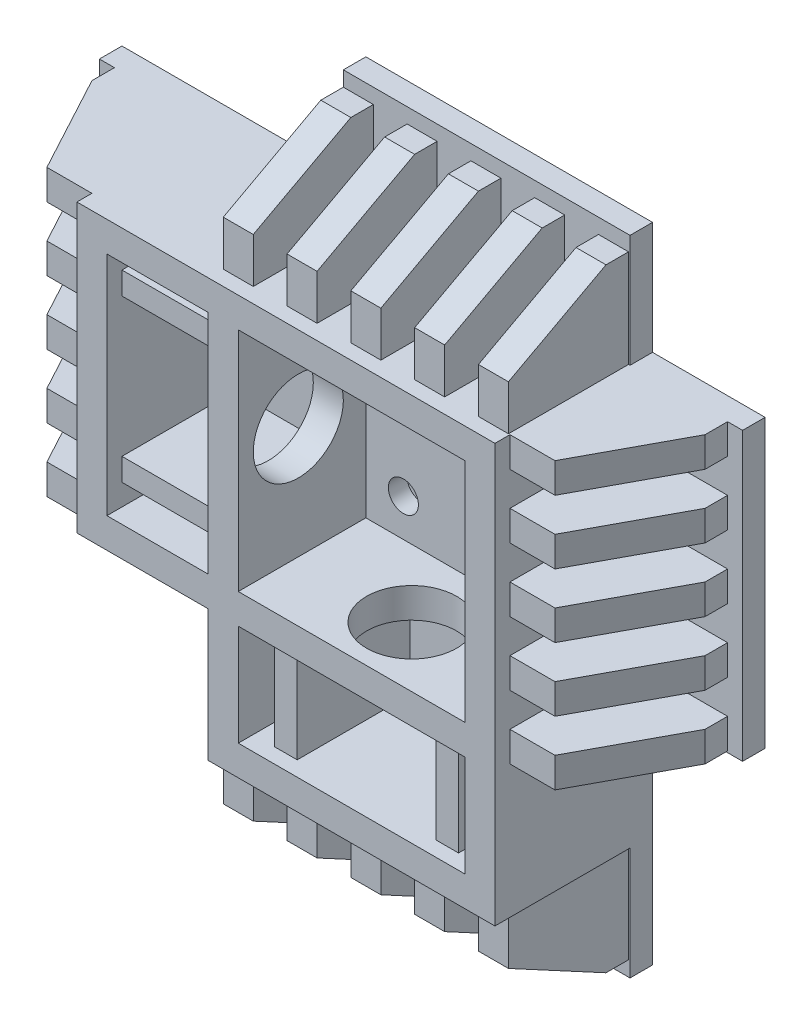
SolidWorks part; units mm, degrees
ref_plane "Front Plane" through (0, 0, 0) normal (0, 0, 1) x (1, 0, 0)
ref_plane "Top Plane" through (0, 0, 0) normal (0, 1, 0) x (1, 0, 0)
ref_plane "Right Plane" through (0, 0, 0) normal (1, 0, 0) x (0, 0, -1)
sketch "Sketch1" plane through (0, 0, 0) normal (0, 0, 1) x (1, 0, 0)
  line L0 (278.5, -428.5) -> (278.5, -103.5)
  line L1 (278.5, 428.5) -> (-103.5, 428.5)
  line L2 (428.5, 278.5) -> (428.5, -103.5)
  line L3 (278.5, -428.5) -> (-103.5, -428.5)
  line L4 (-428.5, 278.5) -> (-428.5, -103.5)
  line L5 (428.5, 428.5) -> (-428.5, -428.5) construction
  line L6 (428.5, -428.5) -> (-428.5, 428.5) construction
  line L7 (278.5, -103.5) -> (428.5, -103.5)
  line L8 (-103.5, -103.5) -> (-103.5, -428.5)
  line L9 (-103.5, -103.5) -> (-428.5, -103.5)
  line L10 (-428.5, 278.5) -> (-103.5, 278.5)
  line L11 (-103.5, 278.5) -> (-103.5, 428.5)
  line L12 (278.5, 428.5) -> (278.5, 278.5)
  line L13 (278.5, 278.5) -> (428.5, 278.5)
  point P0 (0, 0)
  dimension "D1" = 857
  dimension "D2" = 857
  dimension "D3" = 325
  dimension "D4" = 150
  dimension "D5" = 325
  dimension "D6" = 150
extrude "Boss-Extrude1" add sketch "Sketch1" along normal blind 30
sketch "Sketch4" plane through (0, 0, 0) normal (0, 0, -1) x (-1, 0, 0)
  line L1 (-278.5, -278.5) -> (103.5, -278.5)
  line L2 (278.5, -103.5) -> (278.5, 278.5)
  line L3 (103.5, 278.5) -> (-278.5, 278.5)
  line L12 (-278.5, -428.5) -> (103.5, -428.5)
  line L13 (103.5, -428.5) -> (103.5, -103.5)
  line L14 (103.5, -103.5) -> (428.5, -103.5)
  line L15 (428.5, -103.5) -> (428.5, 278.5)
  line L16 (428.5, 278.5) -> (103.5, 278.5)
  line L17 (103.5, 278.5) -> (103.5, 428.5)
  line L18 (103.5, 428.5) -> (-278.5, 428.5)
  line L19 (-278.5, 428.5) -> (-278.5, 278.5)
  line L20 (-278.5, 278.5) -> (-428.5, 278.5)
  line L21 (-428.5, 278.5) -> (-428.5, -103.5)
  line L22 (-428.5, -103.5) -> (-278.5, -103.5)
  line L23 (-278.5, -103.5) -> (-278.5, -428.5)
  line L25 (103.5, -278.5) -> (103.5, -103.5)
  line L26 (103.5, -103.5) -> (278.5, -103.5)
  line L28 (278.5, 278.5) -> (103.5, 278.5)
  line L35 (-278.5, 278.5) -> (-278.5, -278.5)
  dimension "D1" = 0
extrude "Boss-Extrude2" add sketch "Sketch4" against normal blind 210
sketch "Sketch6" plane through (0, 0, 210) normal (0, 0, 1) x (1, 0, 0)
  line L0 (-278.5, 278.5) -> (278.5, 278.5) construction
  line L1 (238.5, 238.5) -> (-63.5, 238.5)
  line L2 (238.5, 238.5) -> (238.5, -63.5)
  line L3 (238.5, -63.5) -> (-63.5, -63.5)
  line L4 (-63.5, 238.5) -> (-63.5, -63.5)
  line L5 (238.5, 238.5) -> (-63.5, -63.5) construction
  line L6 (238.5, -63.5) -> (-63.5, 238.5) construction
  line L8 (278.5, 278.5) -> (278.5, -278.5) construction
  line L9 (-278.5, 278.5) -> (-278.5, -103.5) construction
  line L10 (-103.5, -63.5) -> (-238.5, -63.5)
  line L11 (-103.5, -63.5) -> (-103.5, 238.5)
  line L12 (-103.5, 238.5) -> (-238.5, 238.5)
  line L13 (-238.5, -63.5) -> (-238.5, 238.5)
  line L14 (-103.5, -63.5) -> (-238.5, 238.5) construction
  line L15 (-103.5, 238.5) -> (-238.5, -63.5) construction
  line L16 (278.5, -278.5) -> (-103.5, -278.5) construction
  line L17 (238.5, -103.5) -> (-63.5, -103.5)
  line L18 (238.5, -103.5) -> (238.5, -238.5)
  line L19 (238.5, -238.5) -> (-63.5, -238.5)
  line L20 (-63.5, -103.5) -> (-63.5, -238.5)
  line L21 (238.5, -103.5) -> (-63.5, -238.5) construction
  line L22 (238.5, -238.5) -> (-63.5, -103.5) construction
  line L23 (-103.5, -278.5) -> (-103.5, -103.5) construction
  point P0 (87.5, 87.5)
  point P7 (-171, 87.5)
  point P16 (87.5, -171)
  dimension "D1" = 302
  dimension "D2" = 302
  dimension "D3" = 40
  dimension "D4" = 40
  dimension "D5" = 40
  dimension "D6" = 40
  dimension "D7" = 40
  dimension "D8" = 40
  dimension "D9" = 40
  dimension "D10" = 40
extrude "Cut-Extrude3" cut sketch "Sketch6" against normal blind 170
sketch "Sketch7" plane through (-63.5, 0, 0) normal (1, 0, 0) x (0, 0, -1)
  line L0 (-210, 278.5) -> (-210, -278.5) construction
  circle A0 centre (-130, 87.5) radius 60
  dimension "D1" = 120
  dimension "D2" = 80
  dimension "D3" = 151
extrude "Cut-Extrude4" cut sketch "Sketch7" against normal blind 148
sketch "Sketch8" plane through (0, 0, 30) normal (0, 0, 1) x (1, 0, 0)
  line L0 (-278.5, -103.5) -> (-278.5, 278.5) construction
  line L1 (-278.5, 238.5) -> (-408.5, 238.5)
  line L2 (-278.5, 238.5) -> (-278.5, 278.5)
  line L3 (-278.5, 278.5) -> (-408.5, 278.5)
  line L4 (-408.5, 238.5) -> (-408.5, 278.5)
  line L5 (-278.5, 238.5) -> (-408.5, 278.5) construction
  line L6 (-278.5, 278.5) -> (-408.5, 238.5) construction
  line L7 (-278.5, 278.5) -> (-428.5, 278.5) construction
  line L8 (-278.5, 153.5) -> (-278.5, 193.5)
  line L9 (-278.5, 153.5) -> (-408.5, 153.5)
  line L10 (-408.5, 153.5) -> (-408.5, 193.5)
  line L11 (-278.5, 193.5) -> (-408.5, 193.5)
  line L12 (-278.5, 68.5) -> (-278.5, 108.5)
  line L13 (-278.5, 68.5) -> (-408.5, 68.5)
  line L14 (-408.5, 68.5) -> (-408.5, 108.5)
  line L15 (-278.5, 108.5) -> (-408.5, 108.5)
  line L16 (-278.5, -16.5) -> (-278.5, 23.5)
  line L17 (-278.5, -16.5) -> (-408.5, -16.5)
  line L18 (-408.5, -16.5) -> (-408.5, 23.5)
  line L19 (-278.5, 23.5) -> (-408.5, 23.5)
  line L20 (-278.5, -101.5) -> (-278.5, -61.5)
  line L21 (-278.5, -101.5) -> (-408.5, -101.5)
  line L22 (-408.5, -101.5) -> (-408.5, -61.5)
  line L23 (-278.5, -61.5) -> (-408.5, -61.5)
  line L25 (408.5, 153.5) -> (408.5, 193.5)
  line L26 (408.5, 238.5) -> (278.5, 238.5)
  line L27 (408.5, 238.5) -> (408.5, 278.5)
  line L28 (408.5, 278.5) -> (278.5, 278.5)
  line L29 (278.5, 238.5) -> (278.5, 278.5)
  line L30 (408.5, 238.5) -> (278.5, 278.5) construction
  line L31 (408.5, 278.5) -> (278.5, 238.5) construction
  line L32 (408.5, 153.5) -> (278.5, 153.5)
  line L33 (278.5, 153.5) -> (278.5, 193.5)
  line L34 (408.5, 193.5) -> (278.5, 193.5)
  line L35 (408.5, 68.5) -> (408.5, 108.5)
  line L36 (408.5, 68.5) -> (278.5, 68.5)
  line L37 (278.5, 68.5) -> (278.5, 108.5)
  line L38 (408.5, 108.5) -> (278.5, 108.5)
  line L39 (408.5, -16.5) -> (408.5, 23.5)
  line L40 (408.5, -16.5) -> (278.5, -16.5)
  line L41 (278.5, -16.5) -> (278.5, 23.5)
  line L42 (408.5, 23.5) -> (278.5, 23.5)
  line L43 (408.5, -101.5) -> (408.5, -61.5)
  line L44 (408.5, -101.5) -> (278.5, -101.5)
  line L45 (278.5, -101.5) -> (278.5, -61.5)
  line L46 (408.5, -61.5) -> (278.5, -61.5)
  point P0 (-343.5, 258.5)
  point P27 (343.5, 258.5)
  dimension "D1" = 40
  dimension "D2" = 130
  dimension "D4" = 130
  dimension "D5" = 40
  dimension "D3" = 5
  dimension "D6" = 5
extrude "Boss-Extrude3" add sketch "Sketch8" along normal blind 160
sketch "Sketch9" plane through (0, 0, 30) normal (0, 0, 1) x (1, 0, 0)
  line L0 (21.5, -408.5) -> (21.5, -278.5)
  line L1 (-63.5, -408.5) -> (-103.5, -408.5)
  line L2 (-63.5, -408.5) -> (-63.5, -278.5)
  line L3 (-63.5, -278.5) -> (-103.5, -278.5)
  line L4 (-103.5, -408.5) -> (-103.5, -278.5)
  line L5 (-63.5, -408.5) -> (-103.5, -278.5) construction
  line L6 (-63.5, -278.5) -> (-103.5, -408.5) construction
  line L11 (-63.5, 408.5) -> (-103.5, 408.5)
  line L12 (-63.5, 408.5) -> (-63.5, 278.5)
  line L13 (-63.5, 278.5) -> (-103.5, 278.5)
  line L14 (-103.5, 408.5) -> (-103.5, 278.5)
  line L15 (-63.5, 408.5) -> (-103.5, 278.5) construction
  line L16 (-63.5, 278.5) -> (-103.5, 408.5) construction
  line L17 (21.5, -408.5) -> (-18.5, -408.5)
  line L18 (-18.5, -408.5) -> (-18.5, -278.5)
  line L19 (21.5, -278.5) -> (-18.5, -278.5)
  line L20 (21.5, 408.5) -> (21.5, 278.5)
  line L21 (21.5, 408.5) -> (-18.5, 408.5)
  line L22 (-18.5, 408.5) -> (-18.5, 278.5)
  line L23 (21.5, 278.5) -> (-18.5, 278.5)
  line L24 (106.5, -408.5) -> (106.5, -278.5)
  line L25 (106.5, -408.5) -> (66.5, -408.5)
  line L26 (66.5, -408.5) -> (66.5, -278.5)
  line L27 (106.5, -278.5) -> (66.5, -278.5)
  line L28 (106.5, 408.5) -> (106.5, 278.5)
  line L29 (106.5, 408.5) -> (66.5, 408.5)
  line L30 (66.5, 408.5) -> (66.5, 278.5)
  line L31 (106.5, 278.5) -> (66.5, 278.5)
  line L32 (191.5, -408.5) -> (191.5, -278.5)
  line L33 (191.5, -408.5) -> (151.5, -408.5)
  line L34 (151.5, -408.5) -> (151.5, -278.5)
  line L35 (191.5, -278.5) -> (151.5, -278.5)
  line L36 (191.5, 408.5) -> (191.5, 278.5)
  line L37 (191.5, 408.5) -> (151.5, 408.5)
  line L38 (151.5, 408.5) -> (151.5, 278.5)
  line L39 (191.5, 278.5) -> (151.5, 278.5)
  line L40 (276.5, -408.5) -> (276.5, -278.5)
  line L41 (276.5, -408.5) -> (236.5, -408.5)
  line L42 (236.5, -408.5) -> (236.5, -278.5)
  line L43 (276.5, -278.5) -> (236.5, -278.5)
  line L44 (276.5, 408.5) -> (276.5, 278.5)
  line L45 (276.5, 408.5) -> (236.5, 408.5)
  line L46 (236.5, 408.5) -> (236.5, 278.5)
  line L47 (276.5, 278.5) -> (236.5, 278.5)
  point P0 (-83.5, -343.5)
  point P6 (-83.5, 343.5)
  dimension "D1" = 40
  dimension "D2" = 130
  dimension "D3" = 130
  dimension "D4" = 40
  dimension "D5" = 5
extrude "Boss-Extrude4" add sketch "Sketch9" along normal up to surface (160 mm away) up to face at (-343.5, 258.5, 190)
sketch "Sketch10" plane through (0, 0, 40) normal (0, 0, 1) x (1, 0, 0)
  line L0 (-238.5, 238.5) -> (-238.5, -63.5) construction
  line L1 (-103.5, 180) -> (-238.5, 180)
  line L2 (-103.5, 180) -> (-103.5, 210)
  line L3 (-103.5, 210) -> (-238.5, 210)
  line L4 (-238.5, 180) -> (-238.5, 210)
  line L5 (-103.5, 180) -> (-238.5, 210) construction
  line L6 (-103.5, 210) -> (-238.5, 180) construction
  line L7 (-103.5, 238.5) -> (-238.5, 238.5) construction
  line L8 (-103.5, -63.5) -> (-103.5, 238.5) construction
  line L9 (-103.5, -5) -> (-238.5, -5)
  line L10 (-103.5, -5) -> (-103.5, -35)
  line L11 (-103.5, -35) -> (-238.5, -35)
  line L12 (-238.5, -5) -> (-238.5, -35)
  line L13 (-103.5, -5) -> (-238.5, -35) construction
  line L14 (-103.5, -35) -> (-238.5, -5) construction
  line L15 (238.5, -103.5) -> (-63.5, -103.5) construction
  line L16 (-5, -238.5) -> (-35, -238.5)
  line L17 (-5, -238.5) -> (-5, -103.5)
  line L18 (-5, -103.5) -> (-35, -103.5)
  line L19 (-35, -238.5) -> (-35, -103.5)
  line L20 (-5, -238.5) -> (-35, -103.5) construction
  line L21 (-5, -103.5) -> (-35, -238.5) construction
  line L22 (-63.5, -103.5) -> (-63.5, -238.5) construction
  line L23 (-63.5, -238.5) -> (238.5, -238.5) construction
  line L24 (-63.5, -238.5) -> (238.5, -238.5) construction
  line L25 (180, -103.5) -> (210, -103.5)
  line L26 (180, -103.5) -> (180, -238.5)
  line L27 (180, -238.5) -> (210, -238.5)
  line L28 (210, -103.5) -> (210, -238.5)
  line L29 (180, -103.5) -> (210, -238.5) construction
  line L30 (180, -238.5) -> (210, -103.5) construction
  point P0 (-171, 195)
  point P9 (-171, -20)
  point P16 (-20, -171)
  point P27 (195, -171)
  dimension "D1" = 30
  dimension "D2" = 28.5
  dimension "D3" = 185
  dimension "D4" = 30
  dimension "D5" = 28.5
  dimension "D6" = 30
  dimension "D7" = 215
  dimension "D8" = 30
extrude "Boss-Extrude5" add sketch "Sketch10" along normal blind 150
sketch "Sketch11" plane through (0, -101.5, 0) normal (0, -1, 0) x (1, 0, 0)
  line L0 (-338.5, 190) -> (-408.5, 60)
  line L1 (-408.5, 190) -> (-278.5, 190) construction
  line L2 (-408.5, 190) -> (-408.5, 30) construction
  line L3 (-408.5, 60) -> (-408.5, 190)
  line L4 (-408.5, 190) -> (-338.5, 190)
  line L5 (338.5, 190) -> (408.5, 60)
  line L6 (278.5, 190) -> (408.5, 190) construction
  line L7 (408.5, 190) -> (408.5, 30) construction
  line L8 (408.5, 60) -> (408.5, 190)
  line L9 (408.5, 190) -> (338.5, 190)
  dimension "D1" = 60
  dimension "D2" = 30
  dimension "D3" = 60
  dimension "D4" = 30
extrude "Cut-Extrude5" cut sketch "Sketch11" against normal blind 663
sketch "Sketch12" plane through (276.5, 0, 0) normal (1, 0, 0) x (0, 0, -1)
  line L0 (-60, 408.5) -> (-190, 338.5)
  line L1 (-190, 408.5) -> (-30, 408.5) construction
  line L2 (-190, 278.5) -> (-190, 408.5) construction
  line L3 (-190, 338.5) -> (-190, 408.5)
  line L4 (-190, 408.5) -> (-60, 408.5)
  line L5 (-190, -338.5) -> (-60, -408.5)
  line L6 (-190, -408.5) -> (-190, -278.5) construction
  line L7 (-190, -408.5) -> (-30, -408.5) construction
  line L8 (-60, -408.5) -> (-190, -408.5)
  line L9 (-190, -408.5) -> (-190, -338.5)
  dimension "D1" = 60
  dimension "D2" = 30
  dimension "D3" = 30
  dimension "D4" = 60
extrude "Cut-Extrude6" cut sketch "Sketch12" against normal blind 663
sketch "Sketch14" plane through (0, -63.5, 0) normal (0, 1, 0) x (1, 0, 0)
  line L0 (-278.5, -210) -> (278.5, -210) construction
  line L1 (-63.5, -40) -> (-63.5, -210) construction
  circle A0 centre (87.5, -130) radius 60
  dimension "D2" = 120
  dimension "D1" = 80
  dimension "D3" = 151
extrude "Cut-Extrude7" cut sketch "Sketch14" against normal blind 60
sketch "Sketch16" plane through (0, 0, 40) normal (0, 0, 1) x (1, 0, 0)
  circle A1 centre (-13.5, 188.5) radius 13
  circle A2 centre (-13.5, 188.5) radius 13
  circle A3 centre (188.5, 188.5) radius 13
  circle A4 centre (188.5, 188.5) radius 13
  circle A5 centre (-13.5, -13.5) radius 13
  circle A6 centre (-13.5, -13.5) radius 13
  circle A7 centre (188.5, -13.5) radius 13
  circle A8 centre (188.5, -13.5) radius 13
  dimension "D1" = 0
  dimension "D2" = 0
  dimension "D3" = 0
  dimension "D4" = 0
extrude "Cut-Extrude10" cut sketch "Sketch16" against normal blind 40
sketch "Sketch18" plane through (0, 0, 40) normal (0, 0, 1) x (1, 0, 0)
  circle A0 centre (-13.5, 188.5) radius 20
  circle A1 centre (188.5, 188.5) radius 20
  circle A3 centre (-13.5, -13.5) radius 20
  circle A4 centre (188.5, -13.5) radius 20
  dimension "D1" = 40
extrude "Cut-Extrude11" cut sketch "Sketch18" against normal blind 25
ref_plane "Plane1" through (87.5, 0, 0) normal (1, 0, 0) x (0, 0, -1)
sketch "Sketch19" plane through (87.5, 0, 0) normal (1, 0, 0) x (0, 0, -1)
  line L0 (-210, 87.5) -> (-118.8519, 87.5)
  line L1 (-210, 238.5) -> (-210, -63.5) construction
